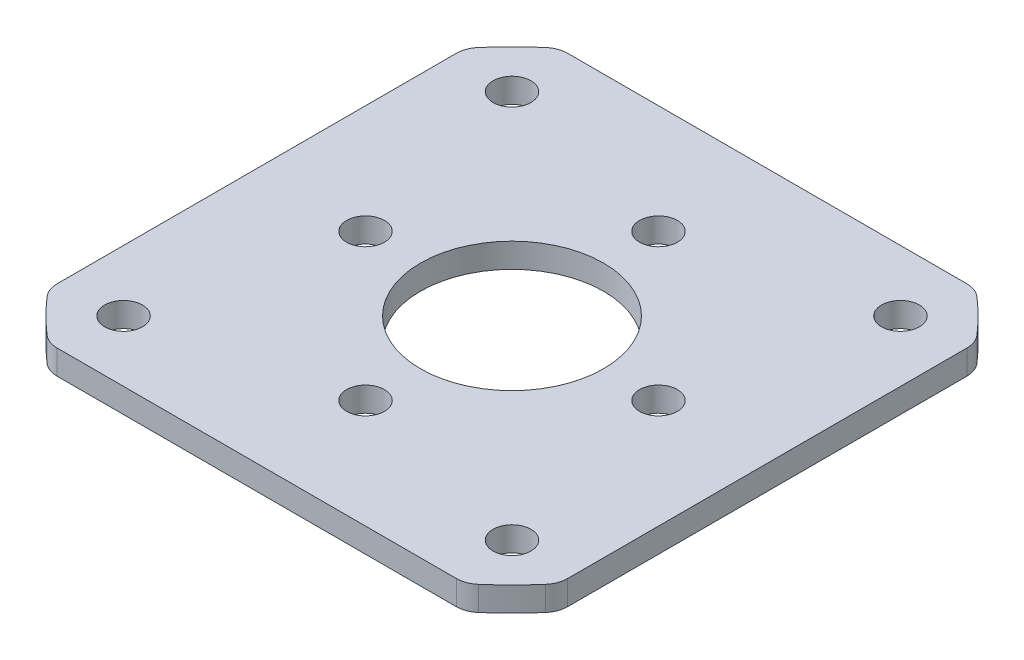
SolidWorks part; units mm, degrees
material "Thornel Mat VMA"
ref_plane "前视基准面" through (0, 0, 0) normal (0, 0, 1) x (1, 0, 0)
ref_plane "上视基准面" through (0, 0, 0) normal (0, 1, 0) x (1, 0, 0)
ref_plane "右视基准面" through (0, 0, 0) normal (1, 0, 0) x (0, 0, -1)
other "Configuration Table"
sketch "草图1" plane through (0, 0, 0) normal (0, 1, 0) x (1, 0, 0)
  line L0 (0, 0) -> (43.0153, 0) construction
  line L1 (0, 0) -> (0, 37.5262) construction
  line L2 (0, 0) -> (31.8198, 31.8198) construction
  line L3 (17.0815, -20.9099) -> (-17.0815, -20.9099)
  line L4 (20.9099, 17.0815) -> (20.9099, -17.0815)
  line L5 (-20.9099, 17.0815) -> (-20.9099, -17.0815)
  line L6 (17.0815, 20.9099) -> (-17.0815, 20.9099)
  circle A0 centre (0, 0) radius 7.5
  circle A1 centre (0, 0) radius 12 construction
  arc A3 (-20.9099, -17.0815) -> (-17.0815, -20.9099) centre (0, 0) ccw
  circle A4 centre (12, 0) radius 1.55
  circle A5 centre (0, 0) radius 22.5 construction
  circle A6 centre (15.9099, 15.9099) radius 1.55
  circle A7 centre (0, -12) radius 1.55
  circle A8 centre (15.9099, -15.9099) radius 1.55
  circle A9 centre (-12, 0) radius 1.55
  circle A10 centre (-15.9099, -15.9099) radius 1.55
  circle A11 centre (0, 12) radius 1.55
  circle A12 centre (-15.9099, 15.9099) radius 1.55
  circle A13 centre (15.9099, 15.9099) radius 3 construction
  circle A14 centre (12, 0) radius 3 construction
  arc A15 (-17.0815, 20.9099) -> (-20.9099, 17.0815) centre (0, 0) ccw
  arc A16 (17.0815, -20.9099) -> (20.9099, -17.0815) centre (0, 0) ccw
  arc A17 (20.9099, 17.0815) -> (17.0815, 20.9099) centre (0, 0) ccw
  point P29 (0, 0)
  dimension "D1" = 24
  dimension "D3" = 15
  dimension "D4" = 3.1
  dimension "D5" = 45
  dimension "D7" = 54
  dimension "D9" = 6
  dimension "D11" = 5
  dimension "D6" = 45
  dimension "D10" = 5
  dimension "D8" = 4
extrude "凸台-拉伸1" add sketch "草图1" along normal blind 2
fillet "圆角1" radius 2 8 edges at (17.0815, 1, 20.9099) (-17.0815, 1, 20.9099) (-20.9099, 1, 17.0815) (-17.0815, 1, -20.9099) (17.0815, 1, -20.9099) (20.9099, 1, -17.0815) (20.9099, 1, 17.0815) (-20.9099, 1, -17.0815)
